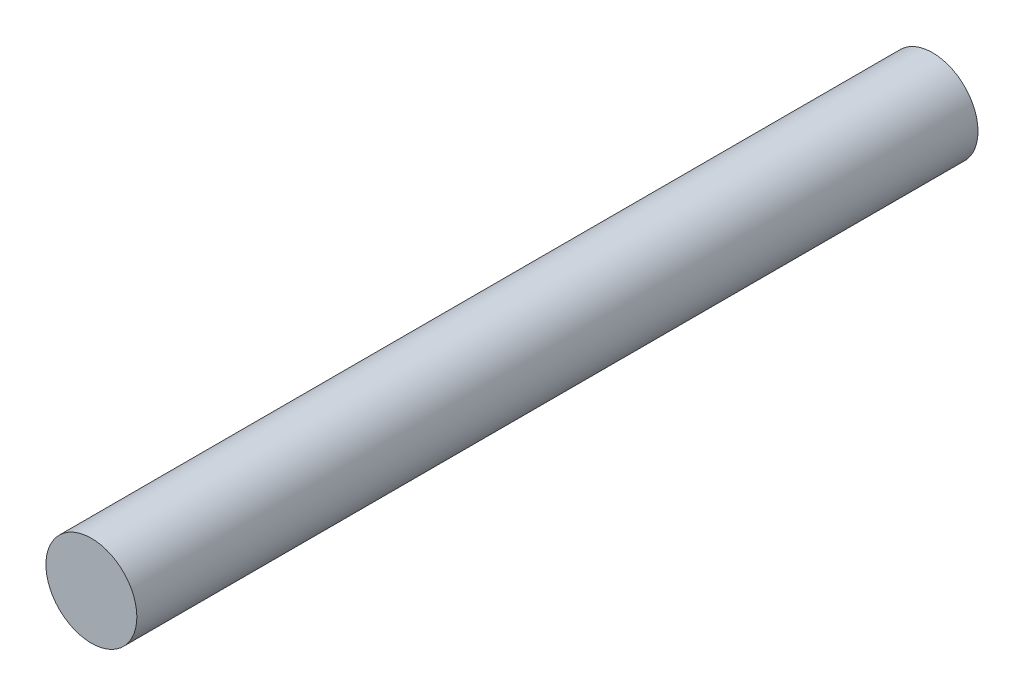
SolidWorks part; units mm, degrees
ref_plane "前视基准面" through (0, 0, 0) normal (0, 0, 1) x (1, 0, 0)
ref_plane "上视基准面" through (0, 0, 0) normal (0, 1, 0) x (1, 0, 0)
ref_plane "右视基准面" through (0, 0, 0) normal (1, 0, 0) x (0, 0, -1)
sketch "草图1" plane through (0, 0, 0) normal (0, 0, 1) x (1, 0, 0)
  circle A0 centre (0, 0) radius 2
  dimension "D1" = 4
extrude "凸台-拉伸1" add sketch "草图1" along normal blind 37
